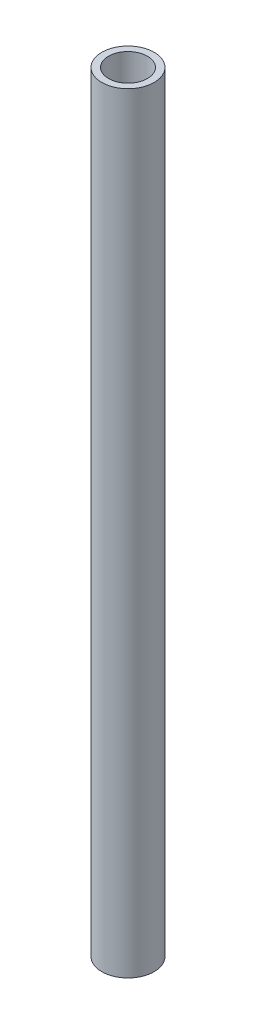
SolidWorks part; units mm, degrees
ref_plane "前基準面" through (0, 0, 0) normal (0, 0, 1) x (1, 0, 0)
ref_plane "上基準面" through (0, 0, 0) normal (0, 1, 0) x (1, 0, 0)
ref_plane "右基準面" through (0, 0, 0) normal (1, 0, 0) x (0, 0, -1)
sketch "草图1" plane through (0, 0, 0) normal (0, 1, 0) x (1, 0, 0)
  circle A0 centre (0, 0) radius 17.5
  dimension "D1" = 35
extrude "凸台-拉伸1" add sketch "草图1" along normal blind 515
shell "抽壳1" thickness 4.5
